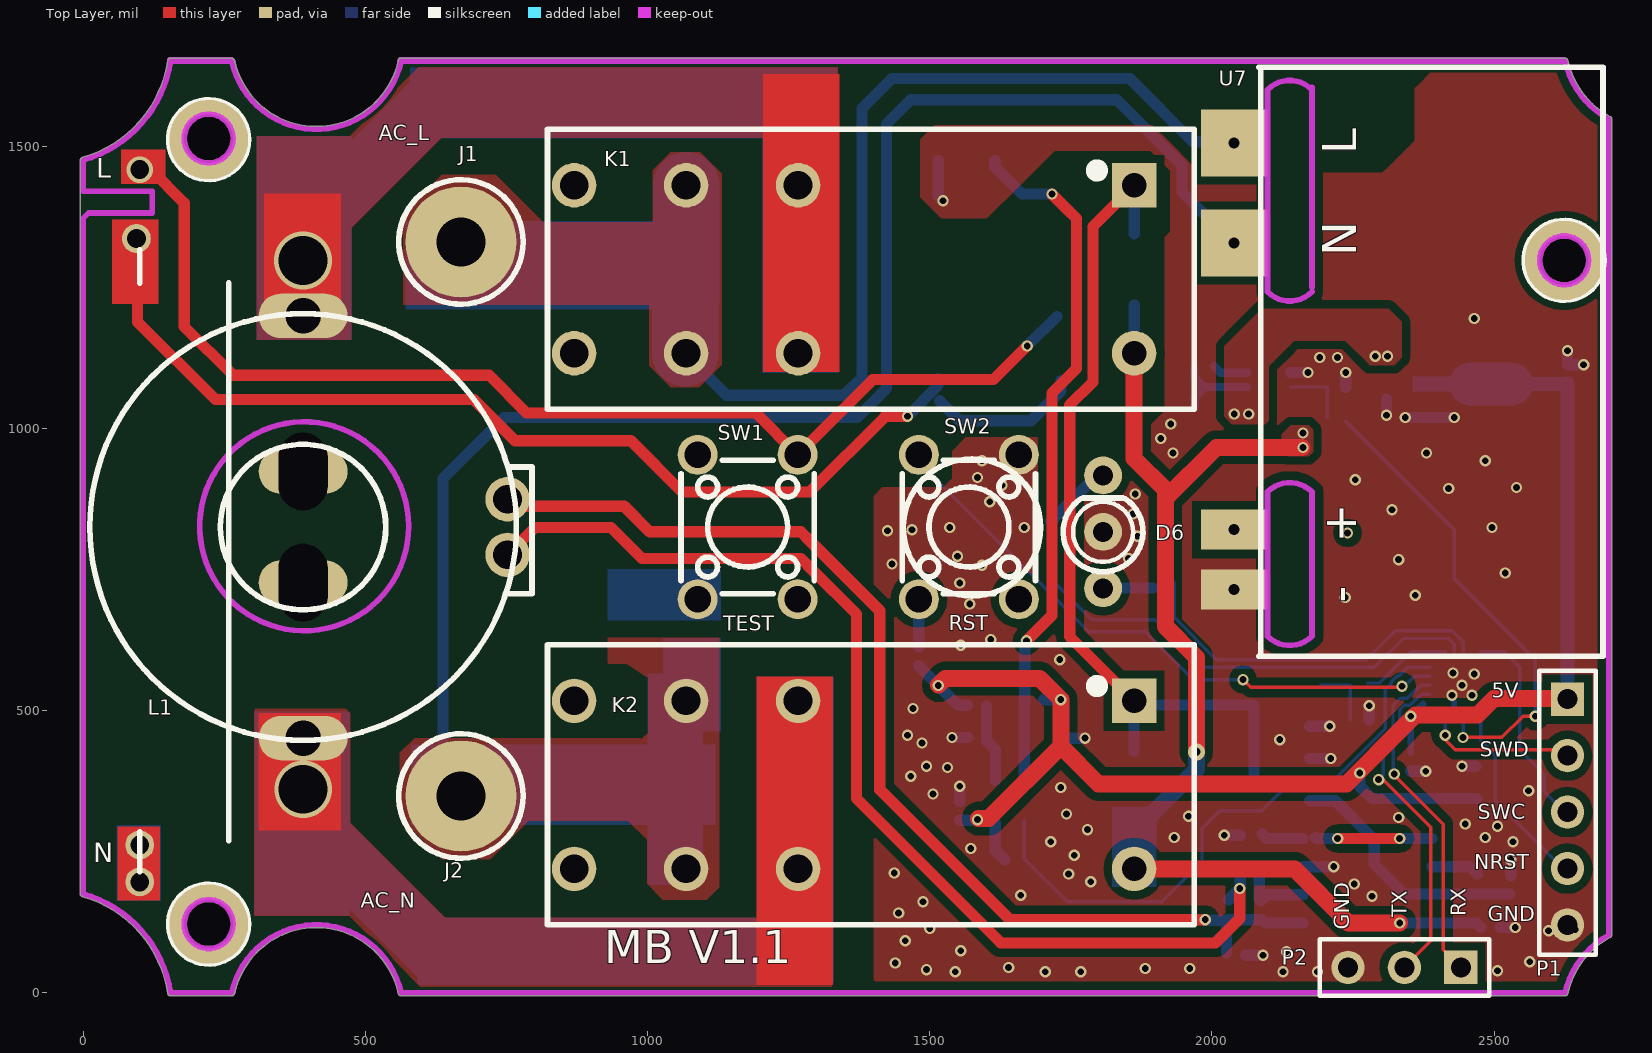
[diagram p0: Top Layer view]
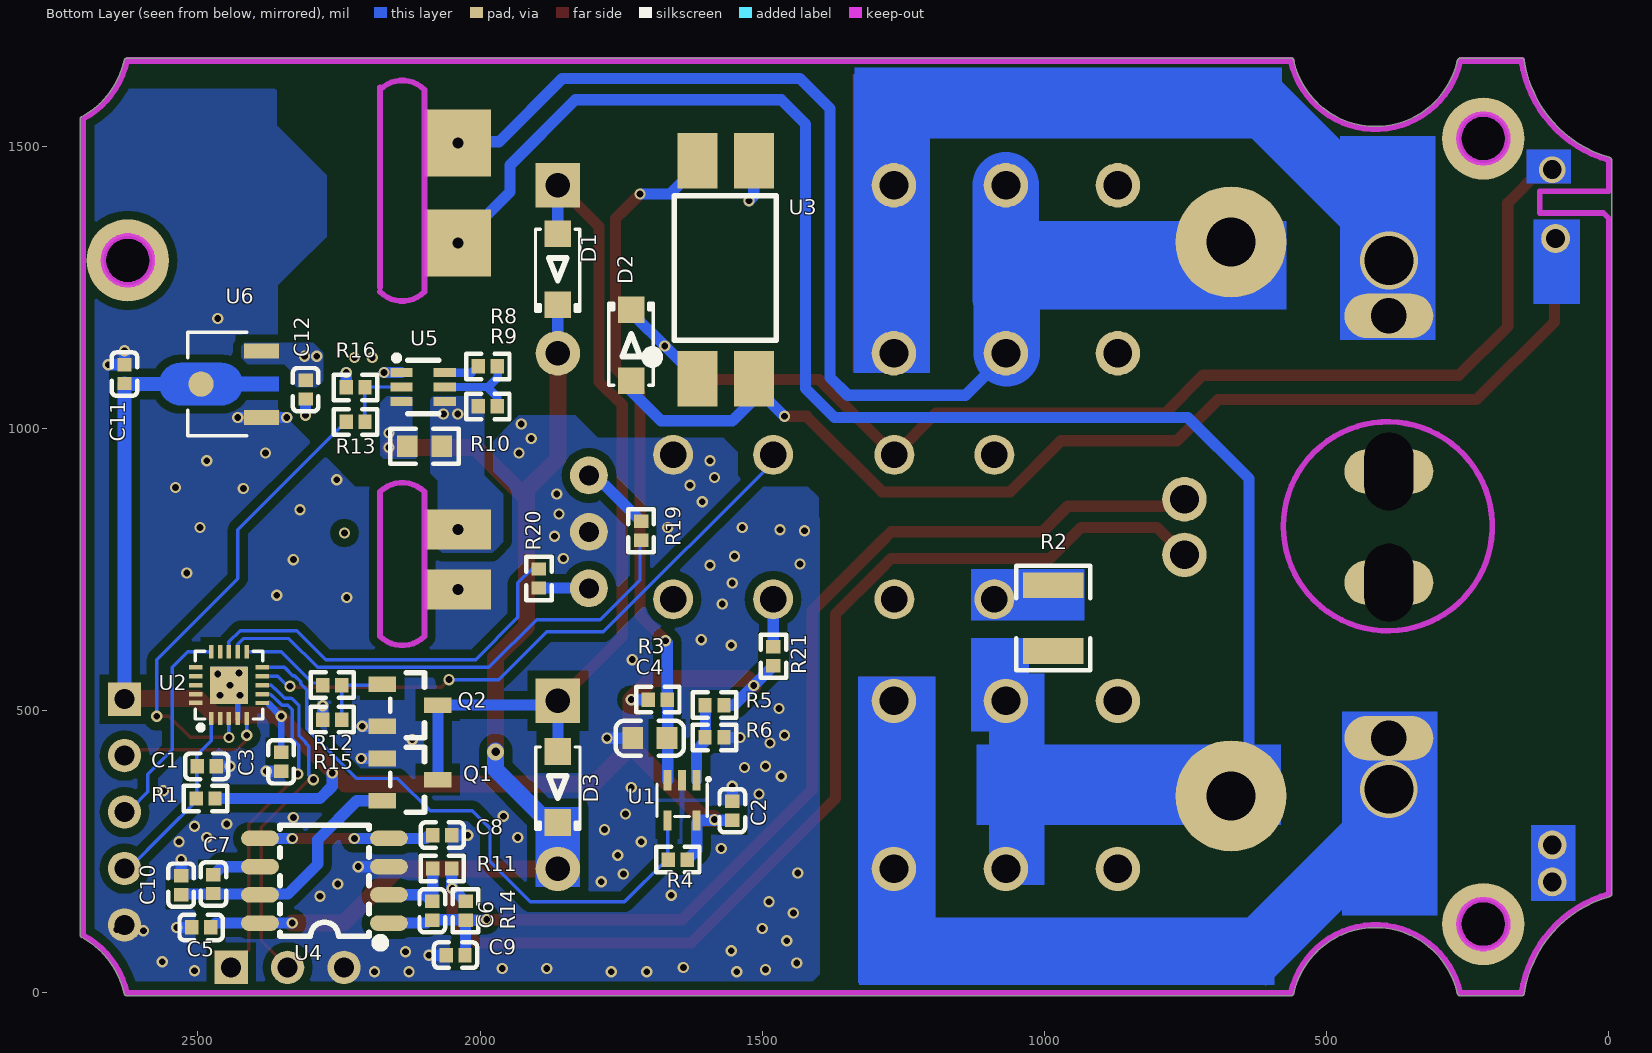
[diagram p1: Bottom Layer view, seen from below]
# Altium PCB MISC89365.PcbDoc
Units mil, origin at the board's own origin, x right, y up, seen from the top; angles counter-clockwise.
Board outline 2713.3 x 1661.01 mil, 2 copper layers (Top Layer, Bottom Layer); 52 components, 39 nets, 172 pads, 143 vias.
Unrouted connection lines stored in the file: 2.

## Layer stack, top to bottom (the 12.6 mil dielectric is the usual default, probably not edited)
Top Layer: signal copper 1.4
Dielectric: dielectric 12.6, FR-4, Dk 4.8
Bottom Layer: signal copper 1.4

## Board outline
-1.37,170.72 cw(c0,175.55) -4.87,176.74 cw(c0,177.93) -5.01,177.93 -5.01,1475.43 cw(c0,1475.43) -1.34,1480.26 ccw(c-59.06,1683.76) 150.03,1651.74 cw(c154.99,1650.98) 154.99,1656 263.38,1656 cw(c263.38,1650.98) 268.28,1652.05 ccw(c413.39,1683.76) 558.49,1652.05 cw(c563.39,1650.98) 563.39,1656 2625.59,1656 cw(c2625.59,1650.98) 2630.49,1652.05 ccw(c2775.59,1683.76) 2705.6,1552.75 cw(c2703.27,1548.32) 2708.28,1548.32 2708.28,102.66 cw(c2703.27,102.66) 2705.6,98.23 cw(c2775.59,-32.78) 2705.63,98.24 2705.6,98.23 ccw(c2775.59,-32.78) 2630.49,-1.07 cw(c2625.59,0) 2625.59,-5.01 563.39,-5.01 cw(c563.39,0) 558.49,-1.07 ccw(c413.39,-32.78) 268.28,-1.07 cw(c263.38,0) 263.38,-5.01 154.99,-5.01 cw(c154.99,0) 150.03,-0.76 ccw(c-59.06,-32.78)

## Design rules (kind name [scope] priority, off if disabled: settings)
Clearance Clearance_1 [inpolygon] p1: gap=6
Clearance [All] p2: gap=6
ComponentClearance [All] p1 off: gap=10 collisioncheckmode=3 verticalgap=10 showdistances=FALSE
HoleSize [All] p1: absolutevalues=TRUE maxlimit=500 minlimit=1 maxpercent=80.000 minpercent=20.000
HoleToHoleClearance [All] p1: gap=0 allowstackedmicrovias=TRUE
MinimumSolderMaskSliver [All] p1: minsoldermaskwidth=0
PlaneConnect [All] p1: planeconnectstyle=Direct reliefexpansion=20 reliefentries=4 reliefconductorwidth=10 reliefairgap=10
PolygonConnect [All] p1: connectstyle=Direct reliefconductorwidth=10 reliefentries=4 polygonreliefangle="90 Angle"
RoutingVias [All] p1: holewidth=12 width=20 viastyle="Through Hole" minholewidth=12 minwidth=20 maxholewidth=12 maxwidth=20
SilkToSilkClearance [All] p1: silktosilkclearance=0
SilkscreenOverComponentPads SilkToSolderMaskClearance [IsPad] p1: minsilkscreentomaskgap=0
SolderMaskExpansion [All] p1: expansion=4
Width [All] p1: maxlimit=300 minlimit=6 preferedwidth=10
21 further rules are at their usual default settings.

## Components (designator, comment, footprint, x,y, rotation, side; value= is the part's Value field where it differs from the comment)
C1 "100nF (104) 10% 50V" 0402_C 2484.25,401.57 r180 bottom
C2 "100nF (104) 10% 50V" 0402_C 1553.15,322.83 r90 bottom
C3 "100nF (104) 10% 50V" 0402_C 2352.36,409.45 r270 bottom
C4 "2.2uF (225) 10% 16V" 0603_C 1699.18,451.5 r0 bottom
C5 "100nF (104) 10% 50V" 0402_C 2494.09,116.14 r180 bottom
C6 "1.0uF (105) 10% 25V" 0402_C 2084.65,145.67 r270 bottom
C7 "47nF (473) 10% 50V" 0402_C 2472.44,192.91 r270 bottom
C8 "47nF (473) 10% 50V" 0402_C 2066.93,279.53 r0 bottom
C9 "47nF (473) 10% 50V" 0402_C 2043.31,66.93 r180 bottom
C10 "47nF (473) 10% 50V" 0402_C 2529.53,190.94 r270 bottom
C11 "1.0uF (105) 10% 25V" 0402_C 2629.92,1096.46 r270 bottom
C12 "1.0uF (105) 10% 25V" 0402_C 2309.06,1068.9 r90 bottom
D1 "A7" SOD-123FL_L2.8-W1.8-LS3.7-RD 1862.39,1282.18 r90 bottom
D2 "A7" SOD-123FL_L2.8-W1.8-LS3.7-RD 1732.28,1147.64 r270 bottom
D3 "A7" SOD-123FL_L2.8-W1.8-LS3.7-RD 1862.2,364.86 r90 bottom
D6 "Common-cathode bicolour LED" "LED 3MM-2P" 1807.09,816.93 r90 top
J1 "Wire solder point, type E" 焊线点E型 669.48,1330.56 r90 top locked
J2 "Wire solder point, type E" 焊线点E型 669.48,349.11 r90 top
K1 "HF115F/012-1ZS3" RELAY-TH_HF115F-012-1ZS3 1366.14,1282.18 r180 top locked
K2 "HF115F/012-1ZS3" RELAY-TH_HF115F-012-1ZS3 1366.14,368.8 r180 top locked
L1 "ZCT56-06N-01" ZCT56-06N-01 389.76,825.49 r90 top locked
P1 "Single-row 2.54 pin header-5P" HDR1X5 2629.92,520.47 r270 top
P2 "Header 3" HDR1X3 2440.94,45.28 r180 top
Q1 "MCR100-6" SOT-23-3_L2.9-W1.3-P1.90-LS2.4-BR 2124.02,377.95 r0 bottom
Q2 "9013" SOT-23(SOT-23-3) 2124.02,509.84 r0 bottom
R1 "10KΩ (1002) ±1%" 0402_R 2486.22,344.49 r180 bottom
R2 "15K 1%" 1210_R 984.44,664.07 r90 bottom
R3 "22KΩ (2202) ±1%" 0402_R 1685.04,519.68 r0 bottom
R4 "10KΩ (1002) ±1%" 0402_R 1649.61,236.22 r180 bottom
R5 "22KΩ (2202) ±1%" 0402_R 1584.65,509.84 r0 bottom
R6 "22KΩ (2202) ±1%" 0402_R 1584.65,452.76 r0 bottom
R8 "1KΩ (1001) ±1%" 0402_R 1986.22,1110.24 r180 bottom
R9 "100KΩ (1003) ±1%" 0402_R 1986.22,1039.37 r180 bottom
R10 "NC" 0603_R 2098.43,968.5 r180 bottom
R11 "100Ω (1000) ±1%" 0402_R 2066.93,220.47 r0 bottom
R12 "470Ω (4700) ±1%" 0402_R 2261.81,545.28 r180 bottom
R13 "1KΩ (1001) ±1%" 0402_R 2220.47,1011.81 r180 bottom
R14 "1KΩ (1001) ±1%" 0402_R 2025.59,145.67 r90 bottom
R15 "10KΩ (1002) ±1%" 0402_R 2261.81,484.25 r180 bottom
R16 "100KΩ (1003) ±1%" 0402_R 2220.47,1072.83 r180 bottom
R19 "3.3KΩ (3301) ±1%" 0402_R 1714.57,818.9 r270 bottom
R20 "3.3KΩ (3301) ±1%" 0402_R 1895.67,734.25 r90 bottom
R21 "10KΩ (1002) ±1%" 0402_R 1480.32,596.46 r270 bottom
SW1 "Through-hole push button 6X6" SW-TH_4P-L6.0-W6.0-P4.50-LS6.5 1177.35,825.49 r90 top locked
SW2 "Through-hole push button 6X6" SW-TH_4P-L6.0-W6.0-P4.50-LS6.5 1569.38,825.47 r90 top locked
U1 "MSLMV331IDCKR" SC-70-5_L2.1-W1.3-P0.65-LS2.3-BL 1642.09,341.26 r0 bottom
U2 "PY32F002BF15U6TR" QFN-20_L3.0-W3.0-P0.40-TL-EP1.7 2444.88,545.28 r90 bottom
U3 "PC817CS" SOP-4_L6.5-W4.6-P2.54-LS10.2-BL 1564.96,1281.5 r180 bottom locked
U4 "GC54123P-A2" SOP-8_L5.0-W4.0-P1.27-LS6.2-BL 2275.59,198.82 r90 bottom
U5 "CJ3439KDW" SOT-363 2100.75,1073.55 r0 bottom
U6 "AMS1117-5.0S" SOT-89-3_L4.5-W2.5-P1.50-LS4.2-BR 2440.94,1078.74 r180 bottom
U7 "5V700mA power module, vertical solder" 5V700mA电源模块竖直焊接 2098.43,671.26 r90 top

## Footprints (in the part's own frame and the unit in brackets; to place one, negate y for a bottom-side part, rotate by r counter-clockwise, add the part's x,y. Pads: shape width x height; smd on the part's side, far side on the other; paste and mask are expansions set on the pad)
5V700mA电源模块竖直焊接 [mm]
  rect 1.8x3 hole 0.5: 1(1.1,1.5) 2(3.8,1.5)
  rect 3x3 hole 0.5: 3(16.7,1.5) 4(21.2,1.5)
  Keep-Out Layer lines w0.254: 14.5,0 ccw(c15.5,-1) 14.5,-2 ; 14.6,0 23.6,0 cw(c22.6,-1) 23.6,-2 ; 14.7,-2 23.7,-2 ; -1,0 ccw(c0,-1) -1,-2 5.5,-2 ccw(c4.5,-1) 5.5,0 -1,0
  silkscreen extent -1.9,-15.1 24.6,0.4
0402_C [mm]
  rect 0.6x0.65 smd mask+0.051: 1(-0.425,0) 2(0.425,0)
  silkscreen extent -0.97,-0.58 0.97,0.58, body extent -0.48,-0.3 0.52,0.3, height 0.2
0402_R [mm]
  rect 0.6x0.65 smd mask+0.051: 1(-0.425,0) 2(0.425,0)
  silkscreen extent -0.97,-0.58 0.97,0.58, body extent -0.57,-0.27 0.58,0.28, height 0.41
0603_C [mm]
  rect 0.93x0.98 smd: 1(-0.77,0) 2(0.77,0)
  silkscreen extent -1.53,-0.79 1.54,0.79, body extent -0.8,-0.4 0.8,0.4, height 0.3
0603_R [mm]
  rect 0.93x0.98 smd: 1(-0.77,0) 2(0.77,0)
  silkscreen extent -1.53,-0.79 1.54,0.79, body extent -0.85,-0.4 0.85,0.4, height 0.56
1210_R [mm]
  rect 1.16x2.72 smd: 1(-1.475,0) 2(1.475,0)
  silkscreen extent -2.35,-1.66 2.36,1.66, body extent -1.6,-1.25 1.6,1.25, height 0.6
HDR1X3 [mm] "Connector; Header; 3 Position"
  rect 1.5x1.5 hole 0.9: 1(0,0)
  round 1.5 hole 0.9: 2(2.54,0) 3(5.08,0)
  silkscreen extent -1.27,-1.27 6.35,1.27
HDR1X5 [mm] "Connector; Header; 6Position"
  rect 1.5x1.5 hole 0.9: 1(0,0)
  round 1.5 hole 0.9: 2(2.54,0) 3(5.08,0) 4(7.62,0) 5(10.16,0)
  silkscreen extent -1.27,-1.27 11.5,1.27, body extent -1.27,-1.27 11.43,1.27, height 7.58
"LED 3MM-2P" [mm]
  round 1.7 hole 0.9: 1(0,0) 2(-2.54,0) 3(2.54,0)
  silkscreen extent -1.8,-1.79 1.52,1.79
QFN-20_L3.0-W3.0-P0.40-TL-EP1.7 [mm]
  rect 0.6x0.2 smd paste-100 mask+0.051: 1(-1.5,0.8) 2(-1.5,0.4) 3(-1.5,0) 4(-1.5,-0.4) 5(-1.5,-0.8) 11(1.5,-0.8) 12(1.5,-0.4) 13(1.5,0) 14(1.5,0.4) 15(1.5,0.8)
  rect 0.2x0.6 smd paste-100 mask+0.051: 6(-0.8,-1.5) 7(-0.4,-1.5) 8(0,-1.5) 9(0.4,-1.5) 10(0.8,-1.5) 16(0.8,1.5) 17(0.4,1.5) 18(0,1.5) 19(-0.4,1.5) 20(-0.8,1.5)
  rect 1.7x1.7 smd paste-100 mask+0.051: 21(0,0)
  silkscreen extent -2,-1.52 1.52,1.52
RELAY-TH_HF115F-012-1ZS3 [mm]
  rect 2x2 hole 1.1: 1(-12.6,-3.78)
  round 2 hole 1.3: 2(2.52,-3.78) 3(7.56,-3.78) 4(12.6,-3.78) 5(12.6,3.78) 6(7.56,3.78) 7(2.52,3.78)
  round 2 hole 1.1: 8(-12.6,3.78)
  silkscreen extent -15.3,-6.3 13.8,6.3
SC-70-5_L2.1-W1.3-P0.65-LS2.3-BL [mil]
  rect 13.8x36.1 smd: 1(-25.6,-35.8) 2(0,-35.8) 3(25.6,-35.8) 4(25.6,35.7) 5(-25.6,35.7)
  silkscreen extent -50,-40 44,29
SOD-123FL_L2.8-W1.8-LS3.7-RD [mm]
  rect 1.2x1.2 smd mask+0.051: 1(-1.6,0) 2(1.6,0)
  silkscreen extent -1.9,-1 1.8,1
SOP-4_L6.5-W4.6-P2.54-LS10.2-BL [mm]
  rect 1.8x2.5 smd: 1(-1.27,-4.9) 2(1.27,-4.9) 3(1.27,4.9) 4(-1.27,4.9)
  silkscreen extent -3.79,-4.42 2.29,3.32
SOP-8_L5.0-W4.0-P1.27-LS6.2-BL [mm]
  oval 0.7x1.7 smd: 1(-1.905,-2.9) 2(-0.635,-2.9) 3(0.635,-2.9) 4(1.905,-2.9) 5(1.905,2.9) 6(0.635,2.9) 7(-0.635,2.9) 8(-1.905,2.9)
  silkscreen extent -2.99,-2.71 2.5,2
SOT-23(SOT-23-3) [mm]
  rect 1.25x0.7 smd: 1(1.25,-0.95) 2(1.25,0.95) 3(-1.25,0)
  silkscreen extent -0.65,-1.46 0.9,1.46, body extent -1.5,-1.5 1.5,1.5, height 1.3
SOT-23-3_L2.9-W1.3-P1.90-LS2.4-BR [mm]
  rect 1.25x0.7 smd: 1(1.25,-0.95) 2(1.25,0.95) 3(-1.25,0)
  silkscreen extent -0.65,-1.46 0.9,1.46
SOT-89-3_L4.5-W2.5-P1.50-LS4.2-BR [mil]
  rect 62x26.5 smd: 1(53.4,-59.1) 3(53.4,59)
  round 44.9 smd: 2(-53.4,0)
  Top Layer region: -89.9,37.4 -16.9,37.4 -15.2,37.3 -13.4,37.2 -11.7,37 -9.9,36.7 -6.5,35.9 -4.9,35.4 -3.2,34.8 -1.6,34.1 0,33.3 1.5,32.5 3,31.6 4.5,30.6 5.9,29.6 7.3,28.5 8.6,27.3 9.8,26.1 12.2,23.5 14.2,20.7 15.2,19.2 16,17.6 16.8,16.1 17.6,13 84.4,13 84.4,-13 17.6,-13 16.8,-16.1 16,-17.7 15.2,-19.2 13.2,-22.2 12.2,-23.5 11,-24.9 9.8,-26.2 8.6,-27.4 7.3,-28.6 5.9,-29.7 4.5,-30.7 3,-31.7 1.5,-32.6 0,-33.4 -3.2,-34.8 -4.9,-35.4 -6.5,-36 -9.9,-36.8 -11.7,-37.1 -13.4,-37.3 -15.2,-37.4 -91.7,-37.4 -93.4,-37.3 -95.2,-37.1 -96.9,-36.8 -100.3,-36 -102,-35.4 -103.6,-34.8 -106.8,-33.4 -108.4,-32.6 -109.9,-31.7 -112.7,-29.7 -114.1,-28.6 -116.7,-26.2 -117.9,-24.9 -119,-23.5 -120.1,-22.2 -121.1,-20.7 -122.9,-17.7 -123.7,-16.1 -124.4,-14.5 -125.6,-11.3 -126.1,-9.6 -126.5,-7.9 -126.8,-6.1 -127.1,-4.4 -127.2,-2.7 -127.3,-0.9 -127.3,0.8 -127.2,2.6 -127.1,4.3 -126.8,6.1 -126.5,7.8 -126.1,9.5 -125.6,11.2 -125,12.9 -124.4,14.5 -123.7,16.1 -122.9,17.6 -122,19.2 -121.1,20.7 -120.1,22.1 -119,23.5 -117.9,24.8 -116.7,26.1 -114.1,28.5 -112.7,29.6 -109.9,31.6 -108.4,32.5 -105.2,34.1 -103.6,34.8 -102,35.4 -100.3,35.9 -96.9,36.7 -95.2,37 -93.4,37.2 -91.7,37.3
  silkscreen extent -77,-92 28,92
SOT-363 [mm]
  rect 1x0.42 smd mask+0.051: 1(0.975,-0.65) 2(0.975,0) 3(0.975,0.65) 4(-0.975,0.65) 5(-0.975,0) 6(-0.975,-0.65)
  silkscreen extent -0.7,-1.43 1.33,1.2
SW-TH_4P-L6.0-W6.0-P4.50-LS6.5 [mm]
  round 1.8 hole 1.2: 1(-3.25,2.25) 2(3.25,2.25) 3(-3.25,-2.25) 4(3.25,-2.25)
  silkscreen extent -3,-3 3,3
ZCT56-06N-01 [mm]
  oval 2x4 hole 1.6: 1(-9.5,0) 2(9.5,0)
  oval 2x4 hole 2.2 slot 3.5 at 0 deg: 3(2.5,0) 4(-2.5,0)
  round 2 hole 1.3: 5(-1.25,-9.2) 6(1.25,-9.2)
  silkscreen extent -9.6,-10.3 9.6,9.6
焊线点E型 [mm]
  round 5 hole 2.2: 1(0,0)
  silkscreen extent -2.8,-2.8 2.8,2.8

## Part data
C1 C2 C3 C5: library part "0402 100nF (104) 10% 50V", "SMD capacitor"
C4: library part "0603 2.2uF (225) 10% 16V", "SMD capacitor"
C6 C11 C12: library part "0402 1.0uF (105) 10% 25V", "SMD capacitor"
C7 C8 C9 C10: library part "0402 47nF (473) 10% 50V", "SMD capacitor"
D1 D2 D3: "General-purpose diode"
D6: library part "LED 3MM-2P共阴", "Bicolour LED red+green"
J1 J2: library part 焊线点E型, "Wire solder joint, hole diameter about 3mm"
K1 K2: "Single changeover (SPDT)"
L1: "Miniature solder-pad zero-sequence sensor"
P1: library part 单排2.54排针-5P
P2: "Header, 3-Pin"
Q1: "0.8A unidirectional thyristor"
Q2: library part "SOT-23 9013", "Transistor"
R1 R4 R15 R21: library part "0402 10KΩ (1002) 1%", "SMD resistor"
R2: library part "1210 15K 1%", "SMD resistor"
R3 R5 R6: library part "0402 22KΩ (2202) 1%", "SMD resistor"
R8 R13 R14: library part "0402 1KΩ (1001) 1%", "SMD resistor"
R9 R16: library part "0402 100KΩ (1003) 1%", "SMD resistor"
R10: library part "0603 0Ω (0R0) 1%", "SMD resistor"
R11: library part "0402 100Ω (1000) 1%", "SMD resistor"
R12: library part "0402 470Ω (4700) 1%", "SMD resistor"
R19 R20: library part "0402 3.3KΩ (3301) 1%", "SMD resistor"
SW1 SW2: library part 直插按键6X6
U1: "Single-channel comparator"
U2: "PUYA M0 microcontroller"
U3: "Optocoupler"
U4: "Leakage protection"
U5: "NMOS+PMOS"
U7: library part 5V700mA电源模块竖直焊接

## Free pads (board coordinates)
  round 145.67 hole 86.61: 0(222.44,122.05) 0(222.44,1513.78) 0(2624.02,1297.93)
  round 51.18 hole 33.46: 1(100.39,196.85) 1(100.39,262.31) 2(94.49,1336.61)

## Via types
v1: diameter 20, hole 12, Top Layer to Bottom Layer, tented both sides, 139 vias
v2: diameter 102.36, hole 86.61, Top Layer to Bottom Layer, tented both sides, 2 vias
v3: diameter 47.24, hole 33.46, Top Layer to Bottom Layer, tented both sides, 1 vias
v4: diameter 30, hole 15, Top Layer to Bottom Layer, tented both sides, 1 vias

## Nets (pads, with @x,y where several pads share a name; then routed paths per layer and width w, separated by ;. In a path a pad name is that pad's centre, name@x,y a point inside that pad or via, vN(x,y) a via of type N, cw(c..) or ccw(c..) an arc to the next point about the centre after c; other vN are vias at no path point)
54123_IN: L1.5 R11.1 R14.2 | length 1948.5
  Top Layer w20: L1.5 800.49,824.8 935.04,824.8 990.16,769.68 1271.65,769.68 1293.31,748.03 1370.08,671.26 1370.08,344.49 1625.98,88.58 2005.91,88.58 2049.21,131.89 v1(2049.21,185.04)
  Bottom Layer w20: R14.2@2029.53,165.35 2050.2,186.02 R11.1
54123_VR: C6.2 C9.2 L1.6 R14.1 U4.1 | length 1960.7
  Top Layer w20: L1.6 764.47,862.2 948.82,862.2 958.66,862.2 1003.94,816.93 1271.65,816.93 1287.4,801.18 1411.42,677.17 1411.42,360.24 1641.73,129.92 v1(1988.19,129.92)
  Bottom Layer w20: v1(1988.19,129.92) 1989.17,128.94 R14.1 C9.2@2025.59,70.87 ; R14.1@2029.53,129.92 2088.58,129.92 2094.69,123.82 U4.1
AC_L: J1.1 K1.3 K1.6 U7.4 | length 1855.6
  Bottom Layer w20: K1.6@1078.74,1120.08 1139.76,1059.06 1348.43,1059.06 1379.92,1090.55 1379.92,1566.93 1433.07,1620.08 1854.33,1620.08 1966.54,1507.87 U7.4@2033.46,1507.87
  Bottom Layer w40: 1066.93,1229.43 1068.5,1231 ; K1.6 K1.6@1082.23,1119.63
  Bottom Layer w118.11: K1.6@1066.93,1133.36 1066.93,1229.43 ; 1068.5,1231 K1.3
AC_N: J2.1 K2.3 K2.6 R2.1 U7.3 | length 2647.2
  Bottom Layer w20: J2.1@655.51,377.95 637.8,395.67 637.8,911.42 746.06,1019.68 1372.05,1019.68 1423.23,1070.87 1423.23,1539.37 1466.54,1582.68 1830.71,1582.68 1946.85,1466.54 1946.85,1419.29 2001.97,1364.17 U7.3@2001.97,1360.24 ; U7.3@2001.97,1356.3 U7.3@2001.97,1360.24 ; U7.3@2025.59,1336.62 U7.3@2001.97,1360.24
  Bottom Layer w40: J2.1@648.07,370.52 J2.1
EN: R13.1 U2.3 | length 838.1
  Top Layer w6: v1(2444.89,452.76) 2513.79,452.76 2551.18,490.16 v1(2572.83,490.16)
  Bottom Layer w6: R13.1 2238.19,1011.81 2429.13,820.87 2429.13,734.25 2572.83,590.55 2572.83,574.8 v1(2572.83,490.16) ; v1(2444.89,452.76) U2.3
GND: C1.2 C2.2 C3.2 C4.2 C5.1 C8.1 C9.1 C10.1 C11.1 C12.1 D6.1 P1.5 P2.3 Q1.1 Q2.2 R6.1 R15.1 R16.1 SW2.4 U1.2 U2.4 U2.21 U3.3 U4.3 U5.1 U6.1 U7.1 | length 747.5
  Bottom Layer w10: U2.4 U2.21@2429.14,515.74
  Bottom Layer w20: U3.3 1514.96,1412.2 v1(1523.62,1403.54) ; v1(1539.37,452.76) R6.1 ; C2.2 v1(1553.15,366.14) ; C4.2 v1(1774.88,451.5) ; v1(2021.65,279.53) C8.1 ; C9.1 v1(2090.55,66.93) ; U5.1 v1(2170,1099.14) ; U4.3 v1(2215.94,223.82) ; Q1.1 v1(2210.63,415.35) ; Q2.2 v1(2208.66,472.44) ; R16.1 v1(2237.2,1099.41) ; R15.1 v1(2278.54,508.86) ; v1(2309.06,1023.62) C12.1 ; v1(2342.56,1019.64) U6.1 v1(2429.09,1019.64) ; C3.2 v1(2378.94,392.72) ; v1(2442.91,401.57) C1.2 ; C5.1 v1(2537.4,116.14) ; C10.1 v1(2529.53,236.22) ; v1(2629.92,1137.8) C11.1 v1(2658.46,1113.19)
  other v1: 1545.28,37.4 1704.72,37.4 1767.72,37.4 2125.98,37.4 2187.01,37.4 2505.91,39.37 1494.09,41.34 1881.89,43.31 1960.63,43.31 1639.76,45.28 1438.98,53.15 2562.99,55.12 2131.89,72.83 1555.12,74.8 1456.69,92.52 2596.46,110.24 2643.7,112.2 1500,114.17 1444.88,141.73 1488.19,161.42 2283.46,171.26 1661.42,173.23 2251.97,192.91 1785.43,196.85 1746.06,210.63 1437.01,212.6 1755.91,244.09 1572.83,255.91 1714.57,267.72 2533.46,267.72 1933.07,275.59 2484.25,275.59 1779.53,289.37 2505.91,295.28 2448.82,299.21 2330.71,311.02 1958.66,312.99 1742.13,316.93 1505.91,352.36 2561.02,358.27 1732.28,364.17 1466.54,383.86 1531.5,399.61 1494.09,401.57 1486.22,442.91 2120.08,448.82 1460.63,456.69 1470.47,503.94 2425.2,527.56 2460.63,527.56 2442.91,545.28 2464.57,564.96 2427.17,566.93 1730.32,590.55 1555.12,616.14 1608.27,625.98 1570.87,688.98 2236.22,700.79 2360.24,704.72 1553.15,726.38 2519.68,744.09 1592.52,757.87 1433.07,759.84 2330.71,767.72 1852.36,769.68 1549.21,773.62 1868.11,809.06 1425.2,818.9 1468.5,820.87 1535.43,824.8 1667.32,824.8 2496.06,824.8 1860.24,848.43 2318.9,856.3 1606.3,870.08 1864.17,883.86 2419.29,893.7 2539.37,895.67 1627.95,899.61 2253.94,909.45 1584.65,913.39 1592.52,942.91 2484.25,942.91 1931.1,956.69 2379.92,956.69 1909.45,982.28 1927.17,1007.87 2190.94,1125.98 2222.44,1125.98 2464.57,1194.88
INPUT: SW2.2 U2.9 | length 1095.1
  Top Layer w6: v1(2055.12,555.12) 2068.9,541.34 2338.58,541.34 v1(2336.61,543.31)
  Bottom Layer w6: SW2.2 1480.8,940.46 1781.5,639.76 1881.89,639.76 1959.64,562.01 1962.6,559.06 1966.54,555.12 v1@2053.15,555.12 ; v1(2336.61,543.31) 2338.58,541.34 2358.25,561.01 U2.9
L: D2.1 L1.3 SW1.4 U3.1 | length 2152
  Top Layer w19.68: v3(100.39,1458.66) 120.17,1458.66 179.13,1399.69 179.13,1181.1 265.75,1094.49 718.89,1094.49 785.82,1027.56 1191.82,1027.56 SW1.4 1399.11,1086.61 1496.06,1086.61 ; 1501.97,1086.61 1496.06,1086.61 ; v1(1672.64,1146.26) 1613,1086.61 1496.06,1086.61
  Bottom Layer w19.68: SW1.4 SW1.4@1266.48,953.99 ; U3.1 1672.63,1146.26 D2.1@1725.2,1198.82
LED1: R19.2 U2.12 | length 883
  Bottom Layer w6: R19.2@1716.54,799.21 1716.54,732.28 1787.4,661.42 1899.61,661.42 1984.25,576.77 2287.4,576.77 2338.58,627.95 2419.29,627.95 2429.14,618.1 U2.12
LED2: R20.2 U2.13 | length 687.1
  Bottom Layer w6: R20.2@1907.48,751.97 1933.07,726.38 1933.07,665.35 2007.87,590.55 2273.62,590.55 2324.8,641.73 2425.2,641.73 2444.89,622.04 U2.13
N: L1.4 pad.1
NetC6_1: C6.1 R11.2 U4.2 | length 133.3
  Bottom Layer w20: C6.1@2083.66,166.34 R11.2 ; C6.1@2086.61,163.39 2097.05,173.82 U4.2
NetC7_1: C7.1 U4.6 | length 86.2
  Bottom Layer w20: U4.6 2457.28,223.82 C7.1@2470.47,210.63
NetC7_2: C7.2 C10.2 Q1.2 U4.7 | length 448.2
  Bottom Layer w20: Q1.2 2218.5,340.55 2287.4,271.65 2287.4,228.35 2340.55,175.2 C10.2@2527.56,175.2
NetC8_2: C8.2 U4.4 U4.5 | length 283.4
  Top Layer w20: v1(2222.64,273.82) v1(2332.48,273.82)
  Bottom Layer w20: C8.2@2088.58,281.5 2096.26,273.82 U4.4 ; U4.4@2183.07,275.59 2184.84,273.82 v1(2222.64,273.82) ; v1(2332.48,273.82) U4.5
NetD2_2: D2.2 pad.2 U3.2 | length 2074.1
  Top Layer w19.68: pad.2@96.46,1360.32 96.46,1188.98 234.25,1051.18 692.13,1051.18 764.96,978.35 970.47,978.35 1061.02,887.8 1287.4,887.8 1421.26,1021.65 v1(1460.63,1021.65)
  Bottom Layer w19.68: v1(1460.63,1021.65) 1514.96,1075.98 U3.2 ; U3.2@1517.72,1049.21 1553.15,1013.78 1679.13,1013.78 1732.28,1066.93 D2.2
NetD6_2: D6.2 R20.1 | length 79.7
  Bottom Layer w20: D6.2@1815.94,717.52 R20.1
NetD6_3: D6.3 R19.1 | length 110
  Bottom Layer w20: R19.1 D6.3@1792.32,913.39
NetK1_2: K1.2 K1.7 L1.2
  other v2: 389.76,1297.93
NetK2_2: K2.2 K2.7 L1.1
  other v2: 389.95,360.92
NetQ2_1: Q2.1 R12.2 R15.2 | length 106.3
  Bottom Layer w6: Q2.1@2192.91,545.28 R12.2 ; R15.2 R12.2@2245.08,538.39
NetR2_2: R2.2 SW1.1 | length 146.4
  Bottom Layer w20: R2.2@948.18,726.08 R2.2@962.37,711.89 ; R2.2@972.63,722.14 1064.16,722.14 SW1.1
NetR5_2: R5.2 R6.2 U1.1 | length 137.5
  Bottom Layer w20: R5.2@1600.39,507.87 1600.39,446.85 1616.49,430.75 U1.1
NetR8_1: R8.1 U5.6 | length 63
  Bottom Layer w15: R8.1@2003.94,1110.24 2015.04,1099.14 U5.6
NetR8_2: R8.2 R9.2 U5.5 | length 157.1
  Bottom Layer w15: R8.2@1968.5,1106.3 1968.5,1090.55 1985.51,1073.55 U5.5 ; R9.2 1969.49,1056.1 1986.22,1072.83
NetR13_2: R13.2 R16.2 U5.2 | length 119
  Bottom Layer w6: U5.2 2204.01,1073.55 2204.01,1020.4 R13.2@2204.72,1019.69
NetR21_1: R21.1 SW2.1 | length 64
  Bottom Layer w20: R21.1 SW2.1@1480.31,677.17
NRST: C1.1 P1.4 R1.1 U2.1 | length 323.3
  Bottom Layer w6: U2.1 2476.39,480.32 2476.38,446.85 2501.97,421.26 2501.97,340.55 2559.06,283.46 P1.4@2620.08,222.44
OUT: R12.1 U2.11 | length 160.6
  Bottom Layer w6: R12.1@2275.59,549.21 2297.24,549.21 2352.36,604.33 U2.11
PC817_OUT: C4.1 R3.1 U1.3 U3.4 | length 1223
  Top Layer w20: v1(1671.26,624.02) 1716.54,669.29 1716.54,1062.99 1759.84,1106.3 1759.84,1372.05 1750,1381.89 ; v1(1716.54,1415.35) 1716.54,1414.96 1749.8,1381.69
  Bottom Layer w20: U3.4 1614.96,1463.78 1663.39,1415.35 v1@1714.57,1415.35 ; U1.3 R3.1@1667.69,518.08 ; R3.1 1668.31,621.06 v1(1671.26,624.02)
SCR_T: D1.2 D3.2 K1.1 K2.1 Q1.3 Q2.3 | length 1430.7
  Top Layer w19.68: K2.1@1836.61,543.31 1748.03,631.89 1748.03,1041.34 1789.37,1082.68 1789.37,1358.17 K1.1
  Bottom Layer w19.68: D3.2 K2.1@1862.2,509.84 ; D1.2 K1.1@1862.39,1407.29 ; K2.1@1891.73,509.84 Q2.3 ; Q1.3 Q2.3
SENSOR_AC: R4.1 U1.4 U2.10 | length 1065.4
  Bottom Layer w6: R4.1@1667.69,236.59 U1.4 ; R4.1@1669.29,236.22 1744.09,161.42 1911.42,161.42 1982.28,232.28 1982.28,291.34 2013.78,322.83 2088.58,322.83 2145.67,379.92 2218.5,379.92 2307.09,468.5 2307.09,537.4 2317.61,547.92 2317.61,551.18 2328.74,562.31 2331.99,562.31 2346.44,576.76 U2.10
SWC: P1.3 U2.15 | length 360.5
  Bottom Layer w6: U2.15 2517.72,604.33 2545.27,576.77 2545.27,431.1 2588.58,387.8 2588.58,356.3 P1.3@2618.11,326.77
SWD: P1.2 U2.5 | length 266.5
  Top Layer w6: v1@2415.35,456.7 v1(2413.39,456.7) 2413.39,448.82 2431.1,431.1 2622.05,431.1 P1.2@2629.92,423.23
  Bottom Layer w6: v1(2413.39,456.7) U2.5
UART_RX: P2.1 U2.7 | length 577.9
  Top Layer w6: v1@2320.87,387.8 2409.45,299.21 2409.45,76.77 P2.1
  Bottom Layer w6: v1(2322.83,387.79) 2320.87,387.79 2320.87,438.98 2332.68,450.79 2332.68,501.97 2340.55,509.84 2350.83,509.84 2367.8,526.81 2369.33,526.81 2372.04,529.52 U2.7
UART_TX: P2.2 U2.8 | length 593.3
  Top Layer w6: v1@2299.21,375.98 2305.12,375.98 2387.8,293.31 2387.8,92.13 P2.2
  Bottom Layer w6: 2303.15,385.83 2303.15,437.01 2308.87,442.72 ; 2308.87,443.95 2320.68,455.76 2320.68,506.94 ; 2320.87,509.84 2332.68,521.65 ; 2335.58,521.84 2345.86,521.84 2362.83,538.81 ; 2363.61,538.81 2370.07,545.27 U2.8
  other v1: 2295.28,377.95
VCC_5V: C2.1 C3.1 C11.2 P1.1 R1.2 R3.2 R4.2 R5.1 R21.2 U1.5 U2.6 U6.2 | length 2755.2
  Top Layer w30: v1@1515.75,545.28 1527.56,557.09 1694.88,557.09 v1(1732.28,519.68) ; v1@1586.61,309.06 1604.33,309.06 1732.28,437.01 ; v1@1732.28,517.72 1732.28,437.01 ; P1.1@2620.08,517.72 2616.14,521.65 2500,521.65 2470.47,492.13 2360.24,492.13 2342.52,474.41 2238.19,370.08 1799.21,370.08 1732.28,437.01
  Bottom Layer w12: C3.1 v1(2352.36,490.16) 2374.02,511.81
  Bottom Layer w20: R21.2 1550.2,509.84 R5.1@1566.93,509.84 ; C2.1 v1@1584.64,306.1 ; v1(1584.64,307.08) v1@1584.64,306.1 ; U1.5@1613.19,306.1 v1@1584.64,306.1 ; U1.5@1616.14,301.18 1616.14,252.95 R4.2 ; R3.2 v1(1732.28,519.68) ; v1(2261.81,389.76) 2261.81,366.14 2283.46,344.49 R1.2
  Bottom Layer w25: 2535.43,1078.74 2624.02,1078.74 C11.2@2629.92,1072.83 ; P1.1@2629.92,531.5 C11.2@2629.92,1072.83 ; C11.2 C11.2@2629.92,1072.83
  other v1: 1515.25,544.78
VCC_12V: C12.2 R9.1 R10.2 U5.4 U6.3 U7.2
  other v1: 2039.37,1025.59 2064.96,1025.59 2289.37,1127.95 2311.02,1127.95
VCC_12VC1: C5.2 D1.1 D3.1 K1.8 K2.8 R10.1 U4.8 U5.3 | length 1948.2
  Top Layer w30: K2.8 2146.16,219.98 2242.13,124.02 v1(2332.68,124.02) ; K1.8 1862.2,946.85 1917.32,891.73 1917.32,649.61 1972.44,594.49 v4(1972.44,427.17) ; 1917.32,875.98 2007.87,966.54 2062.99,966.54 v1@2159.45,966.54
  Bottom Layer w19.68: K1.8@1862.39,1141.92 D1.1 ; v1@2332.87,123.82 U4.8 2468.7,123.82 C5.2@2476.38,116.14
  Bottom Layer w30: D3.1 1878.64,301.87 1972.44,395.67 v4(1972.44,427.17) v4@1972.44,429.13
  other v1: 2161.42,966.54 2161.42,992.13
pads on no net: K1.4 K1.5 K2.4 K2.5 SW1.2 SW1.3 SW2.3 U2.2 U2.14 U2.16 U2.17 U2.18 U2.19 U2.20
copper on no net:
  other v1: 2240.16,814.96

## Polygon pours and split planes (outlines as drawn)
VCC_12V on Top Layer "Bottom Layer-No Net" (solid, remove dead copper): 2021.65,1064.96 2021.65,1027.56 2021.65,1021.65 2029.53,1013.78 2035.43,1007.87 2041.34,1007.87 2094.49,1007.87 2098.43,1011.81 2100.39,1013.78 2100.39,1031.5 2100.39,1110.24 2131.89,1141.73 2145.67,1155.51 2204.72,1155.51 2236.22,1155.51 2275.59,1116.14 2279.53,1112.2 2295.28,1112.2 2322.83,1112.2 2330.71,1120.08 2336.61,1125.98 2336.61,1135.83 2336.61,1188.98 2330.71,1194.88 2312.99,1212.6 2155.51,1212.6 2088.58,1212.6 2045.28,1169.29 2021.65,1145.67 2021.65,1064.96
GND on Top Layer "Bottom Layer-No Net" (solid, remove dead copper, pour order 1013): 1400.38,880.01 1400.38,763.86 1400.38,23.71 1427.94,-3.85 1435.81,-11.73 1477.15,-11.73 2675.97,-11.73 2695.65,7.96 2746.84,59.14 2746.84,104.42 2746.84,1525.68 2685.81,1586.7 2634.63,1637.88 2624.79,1637.88 2394.47,1637.88 2366.91,1610.32 2359.04,1602.45 2359.04,1584.73 2359.04,1509.93 2315.73,1466.62 2301.95,1452.84 2189.75,1452.84 1979.12,1452.84 1924,1507.96 1894.47,1537.49 1754.71,1537.49 1508.65,1537.49 1485.02,1513.86 1483.06,1511.9 1483.06,1468.59 1483.06,1409.53 1488.96,1403.63 1520.46,1372.13 1563.76,1372.13 1601.17,1372.13 1658.25,1429.22 1721.24,1492.21 1825.58,1492.21 1890.54,1492.21 1916.13,1466.62 1925.97,1456.78 1925.97,1393.79 1925.97,1348.51 1916.13,1338.67 1916.13,1185.12 1916.13,1031.58 1892.5,1007.96 1868.88,984.34 1736.99,984.34 1563.76,984.34 1542.11,962.68 1540.14,960.72 1540.14,941.03 1540.14,911.5 1532.27,903.63 1524.39,895.75 1481.09,895.75 1416.13,895.75 1400.38,880.01
NetK2_2 on Top Layer "Top Layer-NetK2_2" (solid, pour order 1011): 303.29,499.22 303.29,137.22 471.29,137.22 599.29,9.22 1326.77,9.22 1326.77,133.22 641.29,133.22 473.29,301.22 473.29,495.22 465.29,503.22 305.29,503.22 305.29,501.22
NetK1_2 on Top Layer "Top Layer-NetK1_2" (solid, pour order 1009): 307.29,1157.22 477.29,1157.22 475.29,1159.22 475.29,1355.22 635.29,1515.22 1336.61,1515.22 1336.61,1641.73 595.8,1641.73 472.12,1518.05 308.14,1518.05 307.29,1518.91
AC_N on Top Layer "Top Layer-AC_N" (solid, pour order 1012): 587.29,451.22 561.29,425.22 561.29,311.22 635.29,237.22 721.29,237.22 789.29,305.22 965.29,305.22 999.29,271.22 999.29,193.22 1027.29,165.22 1105.29,165.22 1127.29,187.22 1127.29,629.22 929.29,629.22 929.29,585.22 931.29,583.22 963.29,583.22 993.29,563.22 1001.29,557.77 1001.29,461.22 989.29,449.22 987.29,451.22
AC_L on Top Layer "Top Layer-AC_L" (solid, pour order 1010): 567.29,1219.22 567.29,1383.22 569.29,1383.22 635.29,1449.22 731.29,1449.22 815.29,1365.22 1009.29,1365.22 1009.29,1457.22 1041.29,1489.22 1093.29,1489.22 1131.29,1451.22 1131.29,1113.22 1091.29,1073.22 1041.29,1073.22 1003.29,1111.22 1003.29,1217.22 1001.29,1219.22
VCC_12VC1 on Top Layer "Bottom Layer-No Net" (solid, remove dead copper, pour order 1014): 2124.02,984.25 2124.02,960.63 2129.92,954.72 2133.86,950.79 2145.67,950.79 2171.26,950.79 2175.2,954.72 2179.13,958.66 2179.13,960.63 2179.13,998.03 2171.26,1005.91 2161.42,1005.91 2139.76,1005.91 2127.95,994.09 2124.02,990.16 2124.02,984.25
VCC_12V on Bottom Layer "Bottom Layer-No Net" (solid, remove dead copper): 1958.66,883.86 1958.66,828.74 1958.66,799.21 1970.47,787.4 1978.35,779.53 1998.03,779.53 2066.93,779.53 2072.83,785.43 2074.8,787.4 2074.8,805.12 2074.8,907.48 2086.61,919.29 2088.58,921.26 2088.58,944.88 2088.58,1051.18 2084.65,1055.12 2082.68,1057.09 2076.77,1057.09 1998.03,1057.09 1994.09,1053.15 1992.13,1051.18 1992.13,1045.28 1992.13,917.32 1958.66,883.86
GND on Bottom Layer "Bottom Layer-No Net" (solid, remove dead copper, pour order 1015): 1397.91,842.08 1397.91,330.26 1397.91,33.02 1433.34,-2.41 1474.68,-43.75 1706.96,-43.75 2716.8,-43.75 2769.95,9.4 2819.17,58.61 2819.17,188.53 2819.17,1495.62 2701.06,1601.87 2628.79,1601.87 2579.05,1601.87 2429.45,1601.87 2392,1601.87 2360.5,1601.87 2360.5,1594.04 2360.5,1538.93 2360.5,1536.96 2281.76,1458.22 2271.92,1448.37 2271.92,1409 2271.92,1340.11 2329.01,1283.02 2358.54,1253.49 2358.54,1155.07 2358.54,1034.99 2334.91,1011.37 2220.74,897.19 2153.81,897.19 2057.36,897.19 2002.24,952.31 1931.37,1023.18 1901.84,1023.18 1830.98,1023.18 1807.36,999.56 1791.61,983.81 1630.19,983.81 1569.17,983.81 1555.39,970.03 1543.58,958.22 1543.58,942.47 1543.58,916.88 1535.7,909 1523.89,897.19 1458.93,897.19 1419.56,897.19 1403.81,881.45 1399.87,877.51 1399.87,842.08
VCC_12VC1 on Bottom Layer "Bottom Layer-No Net" (solid, remove dead copper, pour order 1020): 2120.08,1047.24 2120.08,1017.72 2120.08,1005.91 2114.17,1000 2110.24,996.06 2110.24,982.28 2110.24,950.79 2112.2,948.82 2114.17,946.85 2118.11,946.85 2171.26,946.85 2173.23,948.82 2177.17,952.76 2177.17,960.63 2177.17,1045.28 2167.32,1055.12 2165.35,1057.09 2153.54,1057.09 2124.02,1057.09 2122.05,1055.12 2120.08,1053.15 2120.08,1049.21
VCC_12V on Bottom Layer "Bottom Layer-No Net" (solid, remove dead copper, pour order 1022): 2277.56,1124.02 2277.56,1084.65 2283.46,1078.74 2289.37,1072.83 2297.24,1072.83 2324.8,1072.83 2330.71,1078.74 2332.68,1080.71 2332.68,1086.61 2332.68,1100.39 2338.58,1106.3 2346.46,1114.17 2375.98,1114.17 2411.42,1114.17 2419.29,1122.05 2423.23,1125.98 2423.23,1129.92 2423.23,1145.67 2419.29,1149.61 2417.32,1151.57 2411.42,1151.57 2295.28,1151.57 2281.5,1137.8 2277.56,1133.86 2277.56,1125.98

## Keep-outs
Keep-Out Layer:
  circle w10: c391.73,826.77 r185.08
  circle w10: c2624.02,1297.93 r43.31
  circle w10: c222.44,1513.78 r43.31
  circle w10: c222.44,122.05 r43.31
  lines w10: 0,175.55 cw(c-59.06,-32.78) 154.99,0 263.38,0 cw(c413.39,-32.78) 563.39,0 2625.59,0 cw(c2775.59,-32.78) 2703.27,102.66 2703.27,1548.32 cw(c2775.59,1683.76) 2625.59,1650.98 563.39,1650.98 cw(c413.39,1683.76) 263.38,1650.98 154.99,1650.98 cw(c-59.06,1683.76) 0,1475.43 0,1421.26 ; 0,177.93 0,415.22 ; 0,412.04 0,1242.81 0,1372.05 9.84,1381.89 122.74,1381.89 122.74,1420.57 0,1420.57 ; 153.65,1653.54 262.04,1653.54 ; 562.05,1653.54 2624.25,1653.54 ; 2703.27,179.13 2703.27,416.42 ; 2703.27,413.24 2703.27,1244.01 2703.27,1476.63

## Other copper
Top Layer:
  rectangle net NetK1_2: 320.87,1219.22 456.69,1416.22
  rectangle net NetK2_2: 311.02,287.4 456.69,496.06
  rectangle net L: 66.93,1433.07 145.67,1494.09
  rectangle net NetD2_2: 51.18,1220.47 133.86,1370.08
  region net N: 135.83,163.39 135.83,295.28 61.02,295.28 61.02,163.39
  rectangle net NetK1_2: 1204.72,1100.39 1340.55,1627.95
  rectangle net NetK2_2: 1192.91,13.78 1328.74,561.02
Bottom Layer:
  rectangle net NetK2_2: 1192.91,17.72 1330.71,561.02
  rectangle net L: 66.93,1434.43 145.67,1494.09
  region net N: 137.8,162.96 137.8,297.24 59.06,297.24 59.06,162.96
  region net NetD2_2: 133.86,1220.47 133.86,1370.08 51.18,1370.08 51.18,1220.47
  rectangle net NetK1_2: 1204.72,1100.39 1332.68,1639.76
  rectangle net AC_N: 580.71,297.24 1120.08,440.39
  rectangle net AC_L: 570.87,1210.63 1122.05,1368.11
  rectangle net NetK2_2: 592.52,13.78 1328.74,133.86
  rectangle net NetK1_2: 578.74,1513.78 1336.61,1639.76
  rectangle net NetK1_2: 1202.76,1098.43 1338.58,1627.95
  rectangle net AC_N: 1027.75,463.29 1130.11,628.64
  rectangle net NetR2_2: 929.32,660.14 1130.11,750.69
  rectangle net VCC_12VC1: 1823.02,187.69 1901.76,329.43
  rectangle net NetK1_2: 307.27,1157.19 476.56,1518.4
  region net NetK1_2: 663.57,1543.99 586.07,1621.5 326.77,1362.2 404.28,1284.7
  rectangle net AC_N: 1000.19,191.63 1098.61,565.65
  region net NetK2_2: 608.02,12.06 685.23,89.27 441.13,333.36 363.92,256.16
  rectangle net NetK2_2: 303.34,137.51 472.63,498.72

## Silkscreen, mask and mechanical layers (free items; w line width, h text height)
Top Overlay:
  circle w5.91: c222.44,122.05 r72.83
  circle w5.91: c222.44,1511.81 r72.83
  circle w5.91: c2624.02,1297.93 r72.83
  circle w10: c1574.8,824.7 r121.49
  lines w10: 100.39,214.57 100.39,285.43 ; 100.39,1257.87 100.39,1316.93 ; 257.87,269.68 257.87,1257.87
  text "AC_L" at 523.62,1501.97 h45
  text "L" at 23.62,1433.07 h60
  text "RST" at 1533.46,633.86 h45
  text "TEST" at 1134.04,632.58 h45
  text "5V" at 2496.06,513.78 h45
  text "SWD" at 2474.41,409.45 h45
  text "SWC" at 2470.47,299.21 h45
  text "N" at 17.72,220.47 h60
  text "NRST" at 2464.57,210.63 h45
  text "AC_N" at 492.13,141.73 h45
  text "RX" at 2458.66,135.83 h45 r90
  text "TX" at 2354.33,133.86 h45 r90
  text "GND" at 2488.19,118.11 h45
  text "GND" at 2251.97,112.2 h45 r90
  text "MB V1.1" at 923.23,33.46 h100
Top Solder:
  rectangle: 66.93,1431.1 145.67,1494.09
  rectangle: 51.18,1305.12 135.83,1370.08
  region: 135.83,165.35 135.83,295.28 61.02,295.28 61.02,165.35
  rectangle: 307.29,1157.22 475.29,1359.22
  rectangle: 305.29,293.22 473.29,503.22
Bottom Solder:
  rectangle: 2350.39,1059.06 2423.23,1092.52
  rectangle: 2419.29,1062.99 2421.26,1068.9
  rectangle: 2442.91,1051.18 2568.9,1110.24
  rectangle: 66.93,1433.07 145.67,1494.09
  region: 135.83,163.39 135.83,295.28 61.02,295.28 61.02,163.39
  rectangle: 51.18,1305.12 133.86,1370.08
  region: 403.85,1279.22 684.36,1559.74 596.46,1647.64 315.94,1367.13
  region: 669.11,100.15 381.68,387.58 305.12,311.02 592.55,23.59
  rectangle: 590.55,11.81 1326.77,129.92
  rectangle: 1194.88,11.81 1326.77,559.06
  rectangle: 580.71,1511.81 1340.55,1641.73
  rectangle: 1206.69,1102.36 1340.55,1643.7
  rectangle: 1015.75,1090.55 1122.05,1468.5
  rectangle: 572.83,1218.5 1131.89,1364.17
  rectangle: 1005.91,175.2 1120.08,553.15
  rectangle: 645.67,307.09 1124.02,442.91
  rectangle: 307.27,145.67 468.69,494.78
  rectangle: 311.21,1164.07 472.63,1511.81